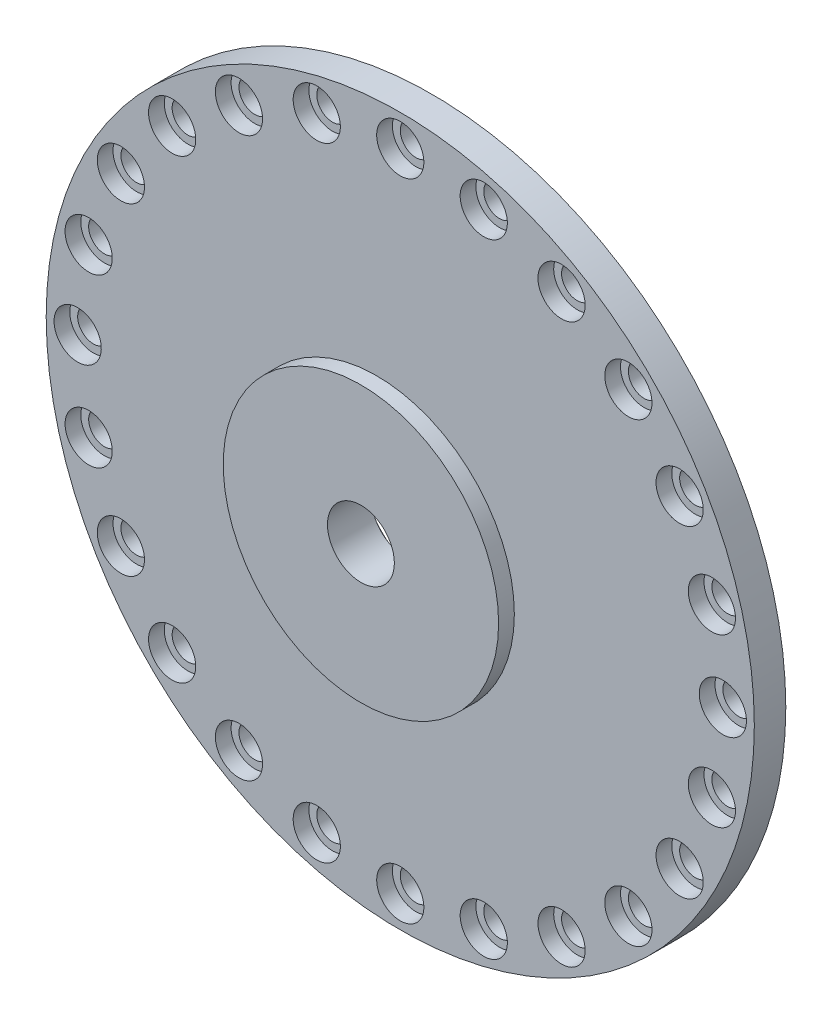
SolidWorks part; units mm, degrees
ref_plane "前视基准面" through (0, 0, 0) normal (0, 0, 1) x (1, 0, 0)
ref_plane "上视基准面" through (0, 0, 0) normal (0, 1, 0) x (1, 0, 0)
ref_plane "右视基准面" through (0, 0, 0) normal (1, 0, 0) x (0, 0, -1)
other "Configuration Table"
sketch "草图1" plane through (0, 0, 0) normal (0, 0, 1) x (1, 0, 0)
  circle A0 centre (0, 0) radius 450
  circle A1 centre (0, 0) radius 42.5
  dimension "D1" = 900
  dimension "D2" = 85
extrude "凸台-拉伸1" add sketch "草图1" along normal mid plane 40
sketch "草图2" plane through (0, 0, 20) normal (0, 0, 1) x (1, 0, 0)
  circle A0 centre (0, 0) radius 410 construction
  circle A1 centre (0, 410) radius 20
  dimension "D1" = 820
  dimension "D2" = 40
sketch "草图5" plane through (0, 0, 20) normal (0, 0, 1) x (1, 0, 0)
  point P0 (0, 410)
hole_wizard "M42 六角头螺栓的柱形沉头孔1" positions "草图5" profile "草图4" counterbore size "M42" standard "GB"
sketch "草图4" plane through (0, 410, 20) normal (1, 0, 0) x (0, -1, 0)
  line L0 (0, 0) -> (0, 62.0172)
  line L1 (0, 62.0172) -> (20, 50)
  line L2 (20, 50) -> (20, 20)
  line L3 (20, 20) -> (30, 20)
  line L4 (30, 20) -> (30, 0)
  line L5 (30, 0) -> (0, 0)
  line L10 (0, 62.0172) -> (-20, 50) construction
  line L11 (0, -6.35) -> (0, 107.95) construction
  dimension "孔直径" = 40
  dimension "孔深度" = 50
  dimension "柱形沉头孔直径" = 60
  dimension "柱形沉头孔深度" = 20
  dimension "导头角度" = 118
sketch "草图6" plane through (0, 0, 0) normal (0, 1, 0) x (1, 0, 0)
  line L0 (0, 0) -> (0, 153.8357)
pattern_circular "阵列(圆周)1" count 24 over 360 about axis through (0, 0, 0) along (0, 0, 1) of "M42 六角头螺栓的柱形沉头孔1"
sketch "草图7" plane through (0, 0, 20) normal (0, 0, 1) x (1, 0, 0)
  circle A0 centre (0, 0) radius 42.5 construction
  circle A1 centre (0, 0) radius 42.5
  circle A2 centre (0, 0) radius 125
  dimension "D1" = 250
extrude "凸台-拉伸2" add sketch "草图7" along normal blind 30
sketch "草图8" plane through (0, 0, 50) normal (0, 0, 1) x (1, 0, 0)
  circle A0 centre (0, 0) radius 175
  circle A1 centre (0, 0) radius 42.5 construction
  circle A2 centre (0, 0) radius 42.5
  dimension "D1" = 350
extrude "凸台-拉伸3" add sketch "草图8" along normal blind 20
sketch "草图9" plane through (0, 0, -20) normal (0, 0, -1) x (-1, 0, 0)
  circle A0 centre (0, 0) radius 90
  dimension "D1" = 180
extrude "切除-拉伸1" cut sketch "草图9" against normal blind 34 contours A0
